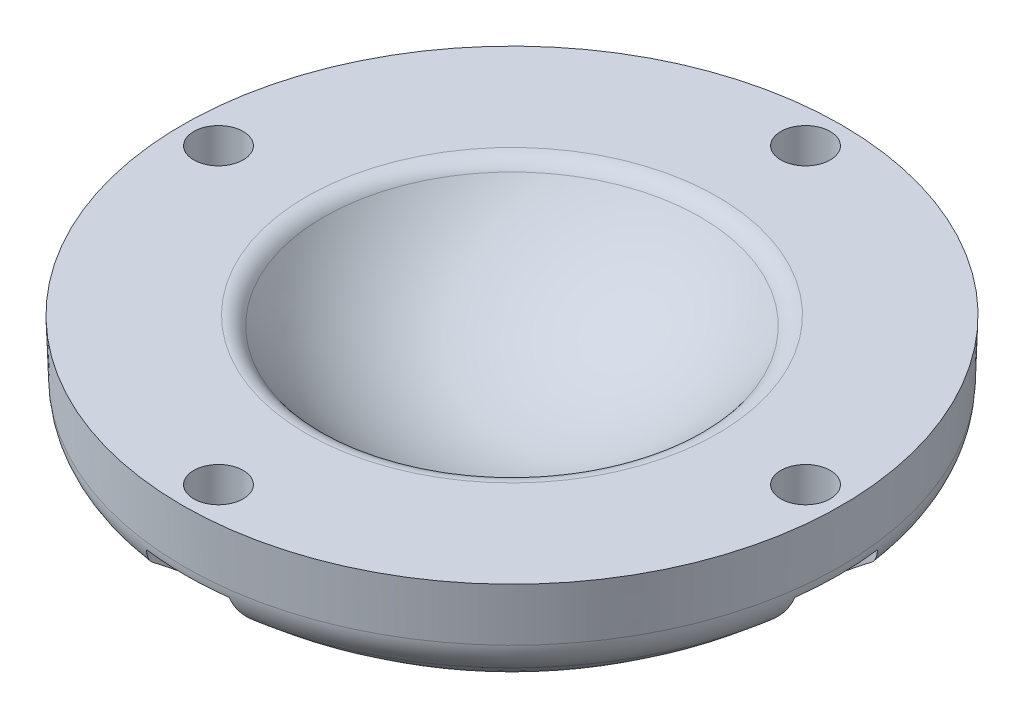
SolidWorks part; units mm, degrees
ref_plane "前视基准面" through (0, 0, 0) normal (0, 0, 1) x (1, 0, 0)
ref_plane "上视基准面" through (0, 0, 0) normal (0, 1, 0) x (1, 0, 0)
ref_plane "右视基准面" through (0, 0, 0) normal (1, 0, 0) x (0, 0, -1)
sketch "草图1" plane through (0, 0, 0) normal (0, 0, 1) x (1, 0, 0)
  line L0 (0, -11) -> (0, -15.5)
  line L1 (15.9081, -8.3029) -> (16, -5.6718)
  line L2 (16, -5.6718) -> (9.9743, -5.6718)
  arc A0 (0, -15.5) -> (15.234, -9.7315) centre (0, 7.5) ccw
  arc A1 (15.234, -9.7315) -> (15.9081, -8.3029) centre (13.9093, -8.2331) ccw
  arc A2 (0, -11) -> (9.1431, -6.1158) centre (0, 0) ccw
  arc A3 (9.9743, -5.6718) -> (9.1431, -6.1158) centre (9.9743, -6.6718) ccw
revolve "旋转1" add sketch "草图1" angle 360 about L0
ref_plane "基准面1" through (0, -15.6718, 0) normal (0, 1, 0) x (1, 0, 0)
hole_wizard "M2 六角头螺栓的柱形沉头孔1" positions "草图4" profile "草图5" counterbore size "M2" standard "GB" end condition through all
sketch "草图4" plane through (0, -15.6718, 0) normal (0, 1, 0) x (1, 0, 0)
  point P0 (-14.25, 0)
  point P8 (0, 14.25)
  point P9 (14.25, 0)
  point P10 (0, -14.25)
  dimension "D1" = 14.25
  dimension "D2" = 4
sketch "草图5" plane through (-14.25, -15.6718, 0) normal (1, 0, 0) x (0, 0, -1)
  line L0 (0, 0) -> (0, 10)
  line L1 (0, 10) -> (1.2, 10)
  line L3 (1.2, 10) -> (1.2, 7)
  line L4 (1.2, 7) -> (2.5, 7)
  line L5 (2.5, 7) -> (2.5, 0)
  line L7 (2.5, 0) -> (0, 0)
  line L11 (0, -6.35) -> (0, 107.95) construction
  dimension "通孔孔直径" = 2.4
  dimension "通孔孔深度" = 10
  dimension "柱形沉头孔直径" = 5
  dimension "柱形沉头孔深度" = 7
